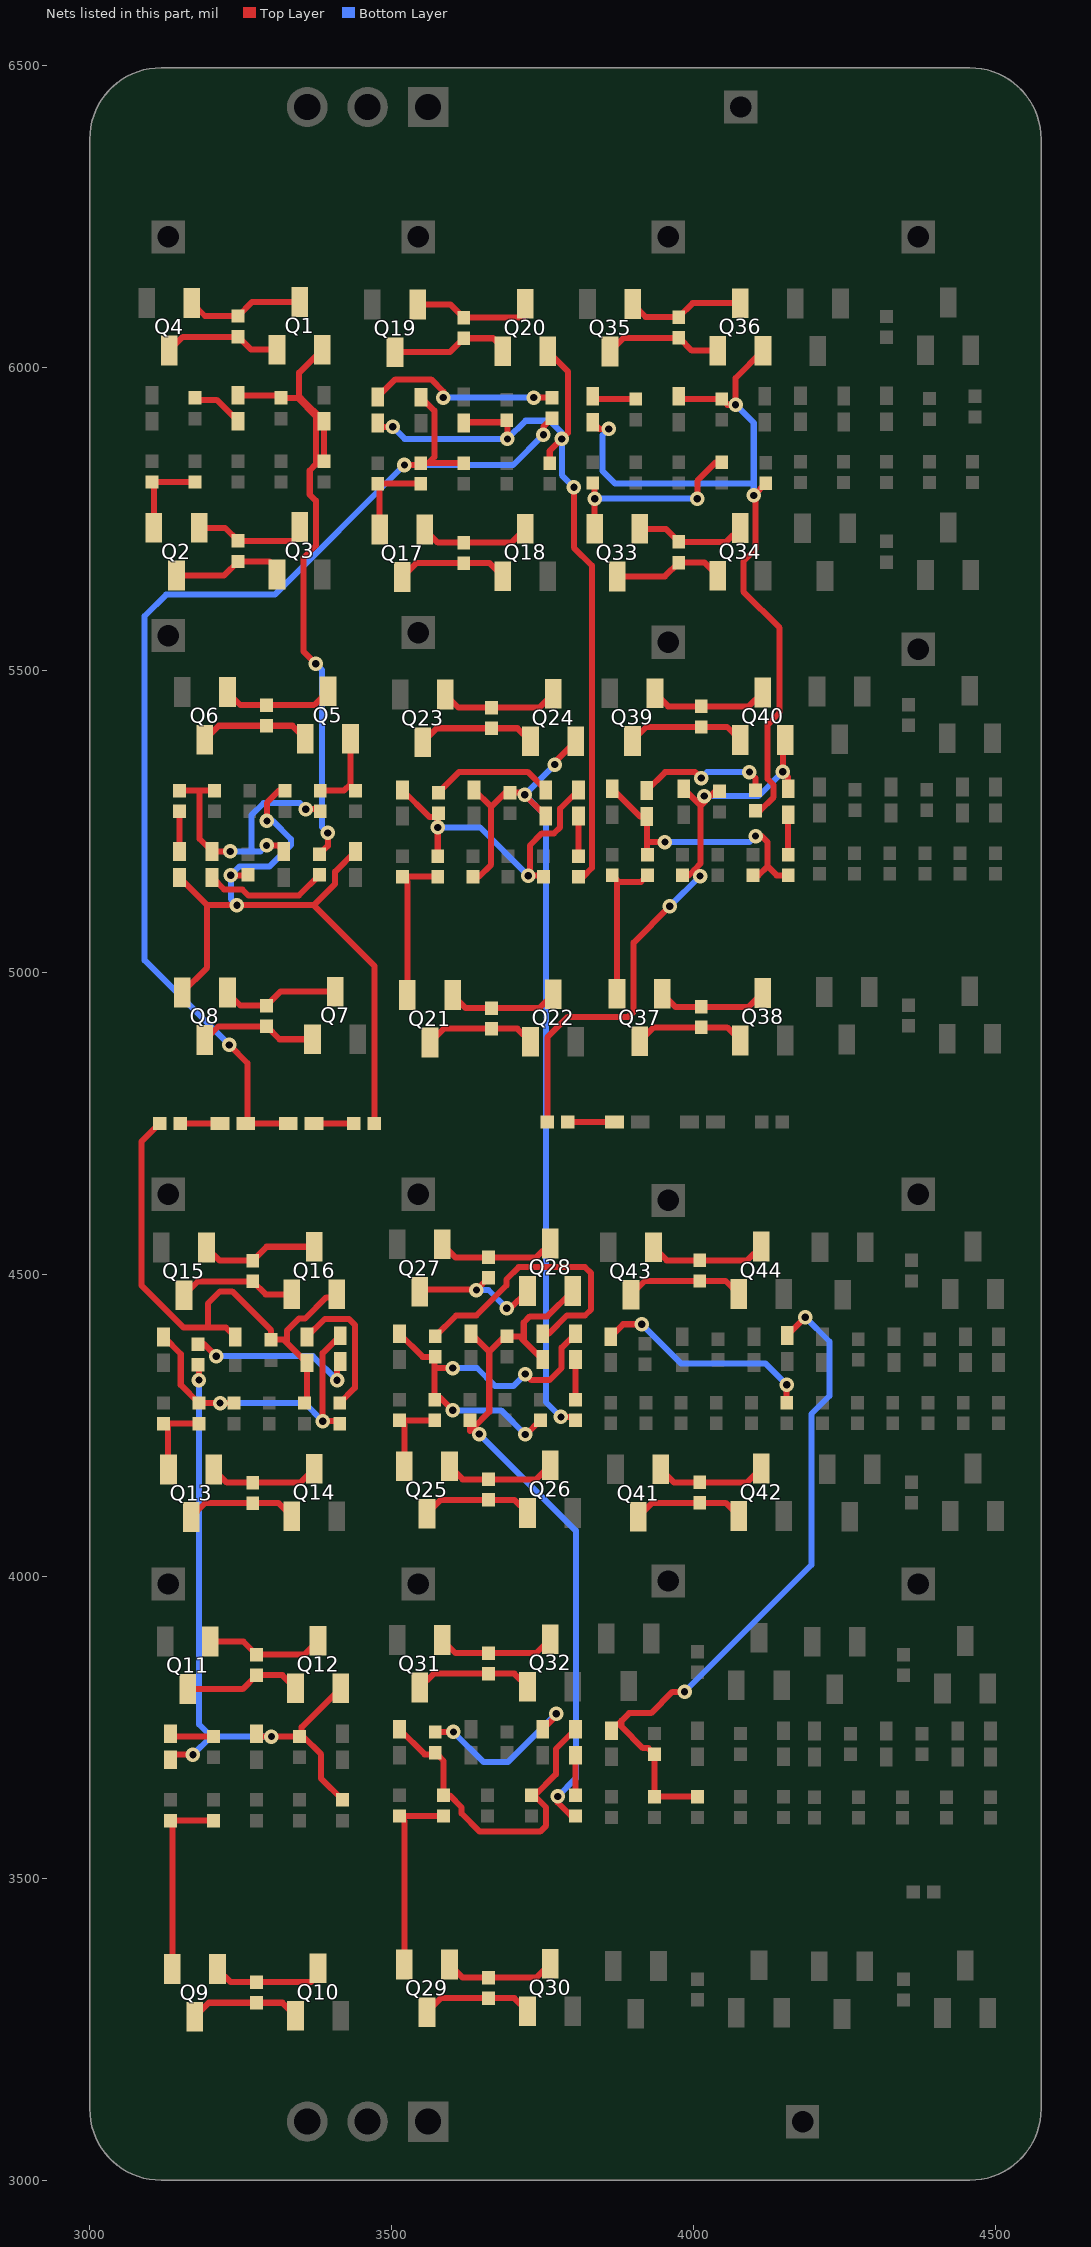
[diagram p0: the nets of this part, all layers, seen from the top]
# Altium PCB MISC61260.pcbdoc (part 2 of 4)
Units mil, origin at the board's own origin, x right, y up, seen from the top; angles counter-clockwise.
Board outline 1574.8 x 3497.01 mil, 2 copper layers (Top Layer, Bottom Layer), stack 62.206 mil thick; 303 components, 159 nets, 654 pads, 177 vias.

## Via types
v1: diameter 24.02, hole 12, Top Layer to Bottom Layer, 177 vias

## Nets (pads, with @x,y where several pads share a name; then routed paths per layer and width w, separated by ;. In a path a pad name is that pad's centre, name@x,y a point inside that pad or via, vN(x,y) a via of type N, cw(c..) or ccw(c..) an arc to the next point about the centre after c; other vN are vias at no path point)
$1N1014: Q2.3 Q3.1 Rb1.2 | length 190.2
  Top Layer w10: Q2.3@3143.57,5656.63 3222.45,5656.63 Rb1.2@3245.47,5679.65 3297.36,5679.65 3309.97,5667.04 Q3.1@3309.97,5658.01
$1N1015: Q2.1 Q3.3 Rb1.1 | length 192.1
  Top Layer w10: Q2.1@3180.97,5735.37 3223.83,5735.37 Rb1.1@3245.47,5713.73 3336.72,5713.73 3347.37,5724.38 Q3.3@3347.37,5736.75
$1N1017: Q1.1 Q4.3 Rb2.2 | length 197.1
  Top Layer w10: Q4.3@3131.67,6028.97 3154.26,6051.57 Rb2.2@3245.9,6051.57 ; Rb2.2@3245.47,6051.99 Rb2.2@3245.9,6051.57 ; Q1.1@3309.97,6030.35 3267.11,6030.35 Rb2.2@3245.9,6051.57
$1N1018: Q1.3 Q4.1 Rb2.1 | length 196.8
  Top Layer w10: Q4.1@3169.07,6107.71 3190.71,6086.07 Rb2.1@3245.47,6086.07 3268.49,6109.09 Q1.3@3347.37,6109.09
$1N1019: C2.2 R1.1 | length 87.1
  Top Layer w10: R1.1@3174.29,5950.38 3177.44,5947.24 3210.12,5947.24 C2.2@3245.47,5911.88
$1N1020: C1.1 C6.2 R6.2 R7.1 Rs3.2 | length 482.1
  Top Layer w10: R6.2@3148.35,5300.22 3181.63,5300.22 ; R7.1@3206.63,5300.22 3181.63,5300.22 ; v1(3232.63,5199.64) C1.1@3202.63,5199.64 3181.63,5220.64 3181.63,5300.22 ; v1(3292.63,5209.64) 3311.19,5209.64 C6.2@3321.19,5199.64 ; v1(3357.63,5269.64) 3377.97,5269.64 Rs3.2@3381.47,5266.14
  Bottom Layer w10: v1(3232.63,5199.64) 3267.63,5199.64 ; v1(3292.63,5209.64) 3282.63,5199.64 3267.63,5199.64 ; v1(3357.63,5269.64) 3347.63,5279.64 3287.63,5279.64 3267.63,5259.64 3267.63,5199.64
$1N1021: C1.2 R5.1 | length 204.5
  Top Layer w10: C1.2@3202.63,5156.72 3222.63,5136.72 3252.63,5136.72 3262.63,5126.72 3346.05,5126.72 R5.1@3380.47,5161.14
$1N1022: C2.1 C5.1 Q1.2 R4.2 R5.2 Rp2.1 | length 1128.8
  Top Layer w10: C2.1@3245.47,5954.8 3312.23,5954.8 Rp2.1@3316.65,5950.38 3344.15,5950.38 ; v1(3374.15,5510.38) 3354.15,5530.38 3354.15,5686.15 3374.15,5706.15 3374.15,5780.38 3364.15,5790.38 3364.15,5830.38 3374.15,5840.38 3374.15,5920.38 3344.15,5950.38 ; R5.2@3380.47,5195.22 3394.15,5208.9 v1(3394.15,5230.38) ; Q1.2@3384.77,6030.35 3346.65,5992.23 3346.65,5950.38 ; R4.2@3387.83,5845.38 C5.1@3387.83,5911.88 3349.33,5950.38 3346.65,5950.38 ; 3344.15,5950.38 3346.65,5950.38
  Bottom Layer w10: v1(3374.15,5510.38) 3384.15,5500.38 3384.15,5240.38 v1(3394.15,5230.38)
$1N1024: Q2.2 Rp1.2 Rs1.1 | length 148.4
  Top Layer w10: Q2.2@3106.17,5735.37 3106.17,5808.25 Rp1.2@3103.12,5811.3 Rs1.1@3174.29,5811.3
$1N1027: Q5.3 Q6.1 Rb3.2 | length 184.9
  Top Layer w10: Q6.1@3227.89,5463.52 3249.53,5441.88 Rb3.2@3292.39,5441.88 3371.27,5441.88 Q5.3@3394.29,5464.9
$1N1028: Q5.1 Q6.3 Rb3.1 | length 184.9
  Top Layer w10: Q6.3@3190.49,5384.77 3213.51,5407.8 Rb3.1@3292.39,5407.8 3335.25,5407.8 Q5.1@3356.89,5386.16
$1N1029: Q5.2 Rp3.2 Rs3.1 | length 144
  Top Layer w10: Rs3.1@3381.47,5300.22 3420.75,5300.22 Rp3.2@3431.69,5311.16 ; Q5.2@3431.69,5386.16 Rp3.2@3431.69,5311.16 ; Rp3.2@3439.75,5300.22 3431.69,5308.28 Rp3.2@3431.69,5311.16
$1N1030: Q7.3 Q8.1 Rb4.2 | length 196.8
  Top Layer w10: Q8.1@3227.89,4966.17 3249.53,4944.53 Rb4.2@3292.39,4944.53 3315.41,4967.55 Q7.3@3406.2,4967.55
$1N1031: Q7.1 Q8.3 Rb4.1 | length 197.1
  Top Layer w10: Q8.3@3190.49,4887.43 3213.09,4910.02 Rb4.1@3292.82,4910.02 ; Rb4.1@3292.39,4910.45 Rb4.1@3292.82,4910.02 ; Q7.1@3368.8,4888.81 3314.03,4888.81 Rb4.1@3292.82,4910.02
$1N1032: C8.2 R6.1 | length 66.5
  Top Layer w10: C8.2@3148.35,5199.64 R6.1@3148.35,5266.14
$1N1034: C7.1 C8.1 Q8.2 R9.2 R10.2 Rp4.1 | length 1258.2
  Top Layer w10: C8.1@3148.35,5156.72 3194.34,5110.72 ; Q8.2@3153.09,4966.17 3194.34,5007.42 3194.34,5110.72 ; v1(3233.19,5160.22) 3260.99,5160.22 Rp4.1@3261.91,5161.14 ; v1(3293.19,5250.22) 3293.19,5280.22 3313.19,5300.22 R9.2@3323.19,5300.22 ; C7.1@3439.75,5199.64 3406.18,5166.08 3406.18,5146.08 3370.83,5110.72 ; R10.2@3471.14,4749.42 3471.14,5010.41 3370.83,5110.72 ; 3194.34,5110.72 v1(3243.69,5110.72) 3370.83,5110.72
  Bottom Layer w10: v1(3233.19,5160.22) v1@3233.69,5160.72 ; v1(3243.69,5110.72) 3233.69,5120.72 v1@3233.69,5160.72 ; v1(3293.19,5250.22) 3303.19,5250.22 3333.19,5220.22 3333.19,5210.22 3297.83,5174.86 3247.83,5174.86 v1@3233.69,5160.72
$1N1124: C9.2 R10.1 | length 65.7
  Top Layer w10: C9.2@3371.34,4749.42 R10.1@3437.06,4749.42
$1N2176: Q9.3 Q10.1 Rb5.2 | length 184.9
  Top Layer w10: Q9.3@3174.06,3270.77 3197.08,3293.79 Rb5.2@3275.95,3293.79 3318.81,3293.79 Q10.1@3340.45,3272.15
$1N2177: Q9.1 Q10.3 Rb5.1 | length 191.4
  Top Layer w10: Q9.1@3211.46,3349.51 3233.1,3327.87 Rb5.1@3275.95,3327.87 3365.87,3327.87 3377.85,3339.86 Q10.3@3377.85,3350.89
$1N2179: Q11.3 Q12.1 Rb6.2 | length 196.8
  Top Layer w10: Q11.3@3162.15,3813.12 3252.93,3813.12 Rb6.2@3275.95,3836.14 3318.81,3836.14 Q12.1@3340.45,3814.5
$1N2180: Q11.1 Q12.3 Rb6.1 | length 196.8
  Top Layer w10: Q11.1@3199.55,3891.86 3254.31,3891.86 Rb6.1@3275.95,3870.22 3354.83,3870.22 Q12.3@3377.85,3893.24
$1N2181: C12.2 R11.1 | length 73
  Top Layer w10: C12.2@3133.6,3738.95 3138.02,3734.53 R11.1@3204.78,3734.53
$1N2182: C13.1 C14.2 R15.2 R16.1 Rs7.2 | length 557.5
  Top Layer w10: C14.2@3122.33,4396.03 3150.61,4367.75 3150.61,4316.61 Rs7.2@3180.61,4286.61 v1(3215.61,4286.61) R16.1@3238.89,4286.61 ; R15.2@3413.73,4252.53 3409.65,4256.61 v1(3385.61,4256.61) 3385.61,4369.08 C13.1@3414.58,4398.05
  Bottom Layer w10: v1(3215.61,4286.61) 3355.61,4286.61 v1(3385.61,4256.61)
$1N2183: C13.2 R12.1 | length 288
  Top Layer w10: R12.1@3179.35,4384.11 3189.35,4384.11 v1(3209.35,4364.11) ; v1(3409.35,4324.11) 3409.35,4349.9 C13.2@3414.58,4355.12
  Bottom Layer w10: v1(3209.35,4364.11) 3369.35,4364.11 v1(3409.35,4324.11)
$1N2184: C11.1 C12.1 Q12.2 R12.2 R13.2 Rp6.1 | length 1125.3
  Top Layer w10: C12.1@3133.6,3696.03 3142.1,3704.53 v1(3170.81,3704.53) ; R12.2@3179.35,4350.03 3180.81,4348.57 v1(3180.81,4324.53) ; C11.1@3275.95,3738.95 3280.37,3734.53 v1(3300.81,3734.53) Rp6.1@3347.13,3734.53 Rp6.1@3350.81,3734.53 ; Q12.2@3415.25,3814.5 3350.81,3750.06 Rp6.1@3350.81,3734.53 ; R13.2@3418.31,3629.53 3382.95,3664.89 3382.95,3704.89 3353.31,3734.53 Rp6.1@3350.81,3734.53
  Bottom Layer w10: v1(3170.81,3704.53) 3200.81,3734.53 ; v1(3180.81,4324.53) 3180.81,3754.53 3200.81,3734.53 ; v1(3300.81,3734.53) 3200.81,3734.53
$1N2192: Q9.2 Rp5.2 Rs5.1 | length 318.4
  Top Layer w10: Q9.2@3136.66,3349.51 3136.66,3592.39 Rp5.2@3133.6,3595.45 Rs5.1@3204.78,3595.45
$1N2202: Q13.3 Q14.1 Rb7.2 | length 184.9
  Top Layer w10: Q13.3@3167.79,4097.85 3190.81,4120.87 Rb7.2@3269.68,4120.87 3312.54,4120.87 Q14.1@3334.18,4099.23
$1N2203: Q13.1 Q14.3 Rb7.1 | length 184.9
  Top Layer w10: Q13.1@3205.19,4176.59 3226.83,4154.95 Rb7.1@3269.68,4154.95 3348.56,4154.95 Q14.3@3371.58,4177.97
$1N2204: Q13.2 Rp7.2 Rs7.1 | length 134.4
  Top Layer w10: Rp7.2@3122.33,4252.53 Rp7.2@3129.83,4252.53 ; Q13.2@3130.39,4176.59 3129.83,4177.15 Rp7.2@3129.83,4252.53 ; Rs7.1@3180.61,4252.53 Rp7.2@3129.83,4252.53
$1N2205: Q15.3 Q16.1 Rb8.2 | length 197.1
  Top Layer w10: Q15.3@3155.88,4465.2 3178.47,4487.79 Rb8.2@3270.11,4487.79 ; Rb8.2@3269.68,4488.22 Rb8.2@3270.11,4487.79 ; Q16.1@3334.18,4466.58 3291.32,4466.58 Rb8.2@3270.11,4487.79
$1N2206: Q15.1 Q16.3 Rb8.1 | length 196.8
  Top Layer w10: Q15.1@3193.28,4543.94 3214.92,4522.3 Rb8.1@3269.68,4522.3 3292.71,4545.32 Q16.3@3371.58,4545.32
$1N2207: C16.2 R15.1 | length 235.8
  Top Layer w10: C16.2@3359.45,4396.03 3389.45,4426.03 3428.87,4426.03 3438.87,4416.03 3438.87,4311.75 R15.1@3413.73,4286.61
$1N2216: C15.1 C16.1 Q16.2 R17.2 R18.2 Rp8.1 | length 937.1
  Top Layer w10: R18.2@3115.55,4749.42 3085.55,4719.42 3085.55,4481.37 3155.55,4411.37 3195.55,4411.37 ; C15.1@3240.89,4396.03 3225.55,4411.37 3195.55,4411.37 ; R17.2@3355.45,4286.61 3359.45,4290.61 C16.1@3359.45,4353.11 3326.25,4386.3 ; Q16.2@3408.98,4466.58 3404.06,4461.66 3391.61,4461.66 3356.25,4426.3 3346.25,4426.3 3326.25,4406.3 3326.25,4386.3 ; 3195.55,4411.37 3195.55,4451.37 3215.55,4471.37 3235.55,4471.37 3300.17,4406.75 Rp8.1@3300.17,4391.61 3320.95,4391.61 3326.25,4386.3
$1N2217: C17.2 R18.1 | length 65.7
  Top Layer w10: R18.1@3149.63,4749.42 C17.2@3215.35,4749.42
$1N2218: C9.1 C17.1 C18.2 R19.2 R21.1 Rs9.2 | length 2020.1
  Top Layer w10: v1(3230.92,4879.42) 3260.92,4849.42 C17.1@3260.92,4749.42 ; C17.1@3258.27,4749.42 C17.1@3260.92,4749.42 ; C9.1@3328.42,4749.42 C17.1@3260.92,4749.42 ; v1(3520.92,5839.42) 3544.66,5839.42 Rs9.2@3547.91,5842.67 3560.41,5842.67 ; C18.2@3548.14,5951.61 3570.41,5929.33 3570.41,5852.67 3560.41,5842.67 ; R21.1@3619.09,5842.67 3560.41,5842.67 ; v1(3750.92,5889.42) 3750.92,5902.75 R19.2@3765.17,5917.01
  Bottom Layer w10: v1(3230.92,4879.42) 3090.92,5019.42 3090.92,5589.42 3126.27,5624.77 3306.27,5624.77 v1(3520.92,5839.42) 3700.92,5839.42 v1(3750.92,5889.42)
$1N3184: Q17.3 Q18.1 Rb9.2 | length 184.9
  Top Layer w10: Q17.3@3517.19,5653.91 3540.21,5676.93 Rb9.2@3619.09,5676.93 3661.95,5676.93 Q18.1@3683.59,5655.29
$1N3185: Q17.1 Q18.3 Rb9.1 | length 184.9
  Top Layer w10: Q17.1@3554.59,5732.65 3576.23,5711.01 Rb9.1@3619.09,5711.01 3697.97,5711.01 Q18.3@3720.99,5734.03
$1N3196: Q19.3 Q20.1 Rb10.2 | length 200.2
  Top Layer w10: Q19.3@3505.29,6026.26 3596.07,6026.26 Rb10.2@3619.09,6049.28 3667.73,6049.28 3683.59,6033.42 Q20.1@3683.59,6027.64
$1N3197: Q19.1 Q20.3 Rb10.1 | length 207.6
  Top Layer w10: Q19.1@3542.69,6105 3597.45,6105 Rb10.1@3619.09,6083.36 3716.35,6083.36 3720.99,6088 Q20.3@3720.99,6106.38
$1N3198: C20.2 R19.1 | length 318.7
  Top Layer w10: C20.2@3476.74,5952.09 3505.74,5981.09 3565.17,5981.09 3585.17,5961.09 v1(3585.17,5951.09) ; v1(3735.17,5951.09) R19.1@3765.17,5951.09
  Bottom Layer w10: v1(3585.17,5951.09) v1(3735.17,5951.09)
$1N3199: C19.1 C20.1 Q20.2 R20.2 R22.2 Rp10.1 | length 1420.8
  Top Layer w10: C20.1@3476.74,5909.17 3483.24,5902.67 v1(3501.45,5902.67) ; C19.1@3619.09,5909.17 3620.09,5910.17 Rp10.1@3691.45,5910.17 ; Rp10.1@3690.27,5913.59 3691.45,5912.41 Rp10.1@3691.45,5910.17 ; v1(3691.45,5882.67) Rp10.1@3691.45,5910.17 ; Q20.2@3758.39,6027.64 3791.45,5994.58 3791.45,5892.67 v1(3781.45,5882.67) 3761.45,5862.67 R20.2@3761.45,5842.67 ; v1(3801.45,5802.67) 3801.45,5702.67 3831.45,5672.67 3831.45,5172.67 3816.73,5157.95 R22.2@3809.15,5157.95
  Bottom Layer w10: v1(3501.45,5902.67) 3521.45,5882.67 v1(3691.45,5882.67) 3721.45,5912.67 3761.45,5912.67 3781.45,5892.67 v1(3781.45,5882.67) 3781.45,5822.67 v1(3801.45,5802.67)
$1N3207: Q17.2 Rp9.2 Rs9.1 | length 148.4
  Top Layer w10: Q17.2@3479.79,5732.65 3479.79,5805.53 Rp9.2@3476.74,5808.59 Rs9.1@3547.91,5808.59
$1N4987: C21.1 C22.2 R23.2 R24.1 Rs11.2 | length 543.7
  Top Layer w10: C22.2@3517.75,5301.45 3562.17,5257.03 R23.2@3576.03,5257.03 ; Rs11.2@3576.03,5192.03 v1(3576.03,5239.53) R23.2@3576.03,5257.03 ; R23.2@3577.03,5262.95 3576.03,5261.95 R23.2@3576.03,5257.03 ; v1(3726.03,5159.53) v1@3728.53,5159.53 ; R24.1@3750.87,5157.95 3749.29,5159.53 v1@3728.53,5159.53 ; C21.1@3809.15,5301.45 3778.53,5270.83 3778.53,5239.53 3768.53,5229.53 3748.53,5229.53 3728.53,5209.53 v1@3728.53,5159.53
  Bottom Layer w10: v1(3576.03,5239.53) 3646.03,5239.53 v1(3726.03,5159.53)
$1N4988: C21.2 R22.1 | length 66.5
  Top Layer w10: R22.1@3809.15,5192.03 C21.2@3809.15,5258.53
$1N4990: Q21.3 Q22.1 Rb11.2 | length 184.9
  Top Layer w10: Q21.3@3563.21,4883.27 3586.23,4906.29 Rb11.2@3665.11,4906.29 3707.97,4906.29 Q22.1@3729.61,4884.65
$1N4991: Q21.1 Q22.3 Rb11.1 | length 184.9
  Top Layer w10: Q21.1@3600.61,4962.01 3622.25,4940.37 Rb11.1@3665.11,4940.37 3743.99,4940.37 Q22.3@3767.01,4963.39
$1N4992: Q21.2 Rp11.2 Rs11.1 | length 257.6
  Top Layer w10: Q21.2@3525.81,4962.01 3525.81,5149.89 Rp11.2@3517.75,5157.95 Rs11.1@3576.03,5157.95
$1N5269: Q23.3 Q24.1 Rb12.2 | length 196.8
  Top Layer w10: Q23.3@3551.3,5380.62 3574.32,5403.64 Rb12.2@3665.11,5403.64 3707.97,5403.64 Q24.1@3729.61,5382
$1N5270: Q23.1 Q24.3 Rb12.1 | length 196.8
  Top Layer w10: Q23.1@3588.7,5459.36 3610.34,5437.72 Rb12.1@3665.11,5437.72 3743.99,5437.72 Q24.3@3767.01,5460.74
$1N5271: C24.2 R23.1 | length 204.5
  Top Layer w10: R23.1@3577.03,5297.03 3611.45,5331.45 3724.87,5331.45 C24.2@3754.87,5301.45
$1N5273: C23.1 C24.1 Q24.2 R25.2 R26.2 Rp12.1 | length 1494.6
  Top Layer w10: R25.2@3634.31,5157.95 3644.31,5157.95 3664.31,5177.95 3664.31,5273.45 ; C23.1@3636.31,5301.45 3664.31,5273.45 ; C24.1@3754.87,5258.53 3716.37,5297.03 Rp12.1@3695.59,5297.03 3687.89,5297.03 3664.31,5273.45 ; v1(3769.91,5343.5) 3769.91,5347.51 Q24.2@3804.41,5382 ; v1(3779.91,4263.5) 3798.61,4263.5 R26.2@3804.15,4257.95
  Bottom Layer w10: v1(3769.91,5343.5) v1(3719.91,5293.5) 3755.26,5258.14 3755.26,4288.14 v1(3779.91,4263.5)
$1N5842: C25.1 C26.2 R27.2 R28.1 Rs13.2 | length 665.6
  Top Layer w10: C26.2@3512.75,4401.45 3551.25,4362.95 R27.2@3572.03,4362.95 3571.03,4361.95 3571.03,4344.53 ; Rs13.2@3571.03,4292.03 Rs13.2@3571.03,4294.53 ; v1(3601.03,4274.53) 3581.03,4294.53 Rs13.2@3571.03,4294.53 ; v1(3601.03,4344.53) 3571.03,4344.53 ; v1(3721.03,4234.53) 3722.45,4234.53 R28.1@3745.87,4257.95 ; v1(3721.03,4334.53) 3731.03,4324.53 3761.03,4324.53 3781.03,4344.53 3781.03,4378.33 C25.1@3804.15,4401.45 ; Rs13.2@3571.03,4294.53 3571.03,4344.53
  Bottom Layer w10: v1(3601.03,4274.53) 3681.03,4274.53 v1(3721.03,4234.53) ; v1(3601.03,4344.53) 3641.03,4344.53 3671.03,4314.53 3701.03,4314.53 v1(3721.03,4334.53)
$1N5849: C25.2 R26.1 | length 66.5
  Top Layer w10: R26.1@3804.15,4292.03 C25.2@3804.15,4358.53
$1N5850: Q25.3 Q26.1 Rb13.2 | length 184.9
  Top Layer w10: Q25.3@3558.21,4103.27 3581.23,4126.29 Rb13.2@3660.11,4126.29 3702.97,4126.29 Q26.1@3724.61,4104.65
$1N5851: Q25.1 Q26.3 Rb13.1 | length 184.9
  Top Layer w10: Q25.1@3595.61,4182.01 3617.25,4160.37 Rb13.1@3660.11,4160.37 3738.99,4160.37 Q26.3@3762.01,4183.39
$1N5852: Q25.2 Rp13.2 Rs13.1 | length 137.6
  Top Layer w10: Q25.2@3520.81,4182.01 3520.81,4249.89 Rp13.2@3512.75,4257.95 Rs13.1@3571.03,4257.95
$1N5859: Q27.3 Q28.1 Rb14.2 | length 232.8
  Top Layer w10: Q27.3@3546.3,4470.62 3549.88,4474.2 v1@3640.66,4474.2 ; v1(3640.11,4473.64) v1@3640.66,4474.2 ; Rb14.2@3660.11,4493.64 v1@3640.66,4474.2 ; v1(3690.11,4443.64) 3696.25,4443.64 Q28.1@3724.61,4472
  Bottom Layer w10: v1(3640.11,4473.64) 3660.11,4473.64 v1(3690.11,4443.64)
$1N5860: Q27.1 Q28.3 Rb14.1 | length 196.8
  Top Layer w10: Q27.1@3583.7,4549.36 3605.34,4527.72 Rb14.1@3660.11,4527.72 3738.99,4527.72 Q28.3@3762.01,4550.74
$1N5861: C28.2 R27.1 | length 471.8
  Top Layer w10: R27.1@3572.03,4397.03 3606.45,4431.45 3639.87,4431.45 3689.87,4481.45 3689.87,4491.45 3709.87,4511.45 3819.87,4511.45 3829.87,4501.45 3829.87,4441.45 3819.87,4431.45 3789.87,4431.45 3759.87,4401.45 C28.2@3749.87,4401.45
$1N5868: C27.1 C28.1 Q28.2 R29.2 R30.2 Rp14.1 | length 1194.4
  Top Layer w10: R29.2@3629.31,4257.95 3629.31,4239.95 3634.62,4245.25 ; C27.1@3631.31,4401.45 3661.31,4371.45 ; v1(3644.62,4235.25) 3634.62,4245.25 ; C28.1@3749.87,4358.53 3718.45,4389.96 ; v1(3774.62,3635.25) 3774.62,3625.25 3796.92,3602.95 R30.2@3804.15,3602.95 ; Q28.2@3799.41,4472 3757.36,4429.96 3728.45,4429.96 3718.45,4419.96 3718.45,4389.96 ; 3634.62,4245.25 3661.31,4271.95 3661.31,4371.45 ; 3661.31,4371.45 3686.89,4397.03 Rp14.1@3690.59,4397.03 3711.37,4397.03 3718.45,4389.96
  Bottom Layer w10: v1(3644.62,4235.25) 3804.62,4075.25 3804.62,3665.25 v1(3774.62,3635.25)
$1N6413: C29.1 C30.2 R31.2 R32.1 Rs15.2 | length 561.5
  Top Layer w10: C30.2@3512.75,3746.45 3554.22,3704.99 R31.2@3575,3704.99 ; R31.2@3572.03,3707.95 R31.2@3575,3704.99 ; R32.1@3731.3,3637.03 3735.6,3637.03 R32.1@3736.16,3636.48 ; C29.1@3804.15,3746.45 3771.51,3713.81 3771.51,3671.83 R32.1@3736.16,3636.48 ; R31.2@3575,3704.99 3585.6,3694.38 Rs15.2@3585.6,3637.03 3595.6,3637.03 3615.6,3617.03 3615.6,3607.03 3645.6,3577.03 3745.6,3577.03 3755.6,3587.03 3755.6,3617.03 R32.1@3736.16,3636.48
$1N6420: C29.2 R30.1 | length 66.5
  Top Layer w10: R30.1@3804.15,3637.03 C29.2@3804.15,3703.53
$1N6421: Q29.3 Q30.1 Rb15.2 | length 184.9
  Top Layer w10: Q29.3@3558.21,3278.27 3581.23,3301.29 Rb15.2@3660.11,3301.29 3702.97,3301.29 Q30.1@3724.61,3279.65
$1N6422: Q29.1 Q30.3 Rb15.1 | length 184.9
  Top Layer w10: Q29.1@3595.61,3357.01 3617.25,3335.37 Rb15.1@3660.11,3335.37 3738.99,3335.37 Q30.3@3762.01,3358.39
$1N6423: Q29.2 Rp15.2 Rs15.1 | length 322.1
  Top Layer w10: Q29.2@3520.81,3357.01 3520.81,3594.89 Rp15.2@3512.75,3602.95 Rs15.1@3585.6,3602.95
$1N6430: Q31.3 Q32.1 Rb16.2 | length 196.8
  Top Layer w10: Q31.3@3546.3,3815.62 3569.32,3838.64 Rb16.2@3660.11,3838.64 3702.97,3838.64 Q32.1@3724.61,3817
$1N6431: Q31.1 Q32.3 Rb16.1 | length 196.8
  Top Layer w10: Q31.1@3583.7,3894.36 3605.34,3872.72 Rb16.1@3660.11,3872.72 3738.99,3872.72 Q32.3@3762.01,3895.74
$1N6432: C32.2 R31.1 | length 288.6
  Top Layer w10: R31.1@3572.03,3742.03 v1(3602.03,3742.03) ; C32.2@3749.87,3746.45 3772.03,3768.61 v1(3772.03,3772.03)
  Bottom Layer w10: v1(3602.03,3742.03) 3652.03,3692.03 3692.03,3692.03 v1(3772.03,3772.03)
$1N11298: Q33.3 Q34.1 Rb17.2 | length 184.9
  Top Layer w10: Q33.3@3873.21,5654.93 3952.09,5654.93 Rb17.2@3975.11,5677.95 4017.97,5677.95 Q34.1@4039.61,5656.31
$1N11299: Q33.1 Q34.3 Rb17.1 | length 184.9
  Top Layer w10: Q33.1@3910.61,5733.67 3953.47,5733.67 Rb17.1@3975.11,5712.03 4053.99,5712.03 Q34.3@4077.01,5735.05
$1N11376: Q35.3 Q36.1 Rb18.2 | length 197.1
  Top Layer w10: Q35.3@3861.3,6027.27 3883.9,6049.87 Rb18.2@3975.53,6049.87 ; Rb18.2@3975.11,6050.3 Rb18.2@3975.53,6049.87 ; Q36.1@4039.61,6028.66 3996.75,6028.66 Rb18.2@3975.53,6049.87
$1N11377: Q35.1 Q36.3 Rb18.1 | length 196.8
  Top Layer w10: Q35.1@3898.7,6106.02 3920.34,6084.38 Rb18.1@3975.11,6084.38 3998.13,6107.4 Q36.3@4077.01,6107.4
$1N11378: C35.2 R33.1 | length 73
  Top Layer w10: C35.2@3832.75,5953.1 3837.17,5948.69 R33.1@3903.93,5948.69
$1N11379: C36.1 C37.2 R37.2 R38.1 Rs19.2 | length 459.3
  Top Layer w10: C37.2@3864.83,5303.53 3910.73,5257.62 C36.1@3922.08,5257.62 3922.08,5215.12 ; Rs19.2@3923.11,5194.11 3922.08,5195.14 3922.08,5215.12 ; v1(3952.08,5215.12) 3922.08,5215.12 ; R38.1@4097.95,5160.03 4106.98,5160.03 4122.08,5175.12 ; v1(4102.08,5225.12) 4112.08,5225.12 4122.08,5215.12 4122.08,5175.12 ; R37.2@4156.23,5160.03 4137.17,5160.03 4122.08,5175.12
  Bottom Layer w10: v1(3952.08,5215.12) 4092.08,5215.12 v1(4102.08,5225.12)
$1N11380: C36.2 R34.1 | length 225.1
  Top Layer w10: C36.2@3922.08,5300.55 3952.66,5331.12 4002.08,5331.12 v1(4012.08,5321.12) ; v1(4092.08,5331.12) 4102.08,5321.12 R34.1@4102.08,5301.12
  Bottom Layer w10: v1(4012.08,5321.12) 4022.08,5331.12 v1(4092.08,5331.12)
$1N11381: C34.1 C35.1 Q36.2 R34.2 R35.2 Rp18.1 | length 1348.2
  Top Layer w10: C35.1@3832.75,5910.19 3843.82,5899.12 v1(3859.15,5899.12) ; C34.1@3975.11,5953.1 3979.53,5948.69 Rp18.1@4046.29,5948.69 4055.85,5939.12 v1(4069.15,5939.12) 4069.15,5983.4 Q36.2@4114.41,6028.66 ; v1(4099.15,5789.12) v1@4099.71,5789.68 ; R34.2@4102.08,5267.05 4109.45,5267.05 4132.08,5289.68 4132.08,5309.68 4122.08,5319.68 4122.08,5409.68 4142.08,5429.68 4142.08,5569.68 4082.08,5629.68 4082.08,5679.68 4102.08,5699.68 4102.08,5787.31 v1@4099.71,5789.68 ; R35.2@4119.15,5809.12 v1@4099.71,5789.68
  Bottom Layer w10: v1(3859.15,5899.12) 3849.15,5889.12 3849.15,5829.12 3869.15,5809.12 4099.15,5809.12 ; v1(4069.15,5939.12) 4099.15,5909.12 4099.15,5809.12 ; v1(4099.15,5789.12) 4099.15,5809.12
$1N11383: Q33.2 Rp17.2 Rs17.1 | length 329.8
  Top Layer w10: Rp17.2@3832.75,5809.6 3835.81,5806.55 v1(3835.81,5783.67) Q33.2@3835.81,5733.67 ; v1(4005.81,5783.67) 4005.81,5813.21 4036.29,5843.69 Rs17.1@4046.29,5843.69
  Bottom Layer w10: v1(3835.81,5783.67) v1(4005.81,5783.67)
$1N11439: Q37.3 Q38.1 Rb19.2 | length 184.9
  Top Layer w10: Q37.3@3910.29,4885.35 3933.31,4908.37 Rb19.2@4012.18,4908.37 4055.04,4908.37 Q38.1@4076.68,4886.73
$1N11440: Q37.1 Q38.3 Rb19.1 | length 184.9
  Top Layer w10: Q37.1@3947.69,4964.09 3969.33,4942.45 Rb19.1@4012.18,4942.45 4091.06,4942.45 Q38.3@4114.08,4965.47
$1N11441: Q37.2 Rp19.2 Rs19.1 | length 254
  Top Layer w10: Rp19.2@3864.83,5160.03 3872.89,5151.97 Rp19.2@3872.89,5149.09 ; Q37.2@3872.89,4964.09 Rp19.2@3872.89,5149.09 ; Rs19.1@3923.11,5160.03 3912.17,5149.09 Rp19.2@3872.89,5149.09
$1N11442: Q39.3 Q40.1 Rb20.2 | length 196.8
  Top Layer w10: Q39.3@3898.38,5382.7 3921.4,5405.72 Rb20.2@4012.18,5405.72 4055.04,5405.72 Q40.1@4076.68,5384.08
$1N11443: Q39.1 Q40.3 Rb20.1 | length 196.8
  Top Layer w10: Q39.1@3935.78,5461.44 3957.42,5439.8 Rb20.1@4012.18,5439.8 4091.06,5439.8 Q40.3@4114.08,5462.82
$1N11444: C39.2 R37.1 | length 66.5
  Top Layer w10: R37.1@4156.23,5194.11 C39.2@4156.23,5260.61
$1N11446: C38.1 C39.1 Q40.2 R39.2 R40.2 Rp20.1 | length 1041.7
  Top Layer w10: R40.2@3757.54,4751.59 3757.54,4891.94 3791.47,4925.87 3891.47,4925.87 3900.23,4934.63 3900.23,5048.87 v1(3960.23,5108.87) ; R39.2@3981.39,5160.03 3991.39,5160.03 4000.23,5168.87 ; C38.1@3983.39,5303.53 4011.39,5275.53 ; v1(4010.23,5158.87) 4000.23,5168.87 ; v1(4017.3,5291.44) v1@4027.3,5291.44 ; Rp20.1@4042.67,5299.11 4034.97,5299.11 v1@4027.3,5291.44 ; Q40.2@4151.48,5384.08 4147.3,5379.9 v1(4147.3,5331.44) 4156.23,5322.51 C39.1@4156.23,5303.53 ; 4000.23,5168.87 4011.39,5180.03 4011.39,5275.53 ; 4011.39,5275.53 v1@4027.3,5291.44
  Bottom Layer w10: v1(3960.23,5108.87) v1(4010.23,5158.87) ; v1(4017.3,5291.44) 4107.3,5291.44 v1(4147.3,5331.44)
$1N11447: C40.2 R40.1 | length 76.9
  Top Layer w10: R40.1@3791.62,4751.59 C40.2@3868.5,4751.59
$1N11448: Q41.3 Q42.1 Rb21.2 | length 184.9
  Top Layer w10: Q41.3@3907.79,4098.27 3930.81,4121.29 Rb21.2@4009.68,4121.29 4052.54,4121.29 Q42.1@4074.18,4099.65
$1N11449: Q41.1 Q42.3 Rb21.1 | length 184.9
  Top Layer w10: Q41.1@3945.19,4177.01 3966.83,4155.37 Rb21.1@4009.68,4155.37 4088.56,4155.37 Q42.3@4111.58,4178.39
$1N11450: Q43.3 Q44.1 Rb22.2 | length 196.8
  Top Layer w10: Q43.3@3895.88,4465.62 3918.9,4488.64 Rb22.2@4009.68,4488.64 4052.54,4488.64 Q44.1@4074.18,4467
$1N11451: Q43.1 Q44.3 Rb22.1 | length 196.8
  Top Layer w10: Q43.1@3933.28,4544.36 3954.92,4522.72 Rb22.1@4009.68,4522.72 4088.56,4522.72 Q44.3@4111.58,4545.74
$1N11452: C43.2 R41.1 | length 371.3
  Top Layer w10: C43.2@3862.33,4396.45 3882.91,4417.03 v1(3913.73,4417.03) ; R41.1@4153.73,4287.03 v1(4153.73,4317.03)
  Bottom Layer w10: v1(3913.73,4417.03) 3978.38,4352.39 4118.38,4352.39 v1(4153.73,4317.03)
$1N11453: C44.1 C45.2 R45.2 R46.1 Rs23.2 | length 1151.7
  Top Layer w10: C45.2@3863.6,3743.95 3880.39,3760.74 ; Rs23.2@3934.78,3634.53 Rs23.2@3934.78,3635.45 ; v1(3984.58,3808.47) 3964.58,3808.47 3929.22,3773.11 3892.76,3773.11 3880.39,3760.74 ; R46.1@4005.95,3634.53 4005.03,3635.45 Rs23.2@3934.78,3635.45 ; C44.1@4154.58,4398.47 v1(4184.58,4428.47) ; 3880.39,3760.74 3880.39,3750.74 3915.74,3715.38 3924.84,3715.38 R45.2@3934.78,3705.45 Rs23.2@3934.78,3635.45
  Bottom Layer w10: v1(3984.58,3808.47) 4194.58,4018.47 4194.58,4268.47 4224.58,4298.47 4224.58,4388.47 v1(4184.58,4428.47)